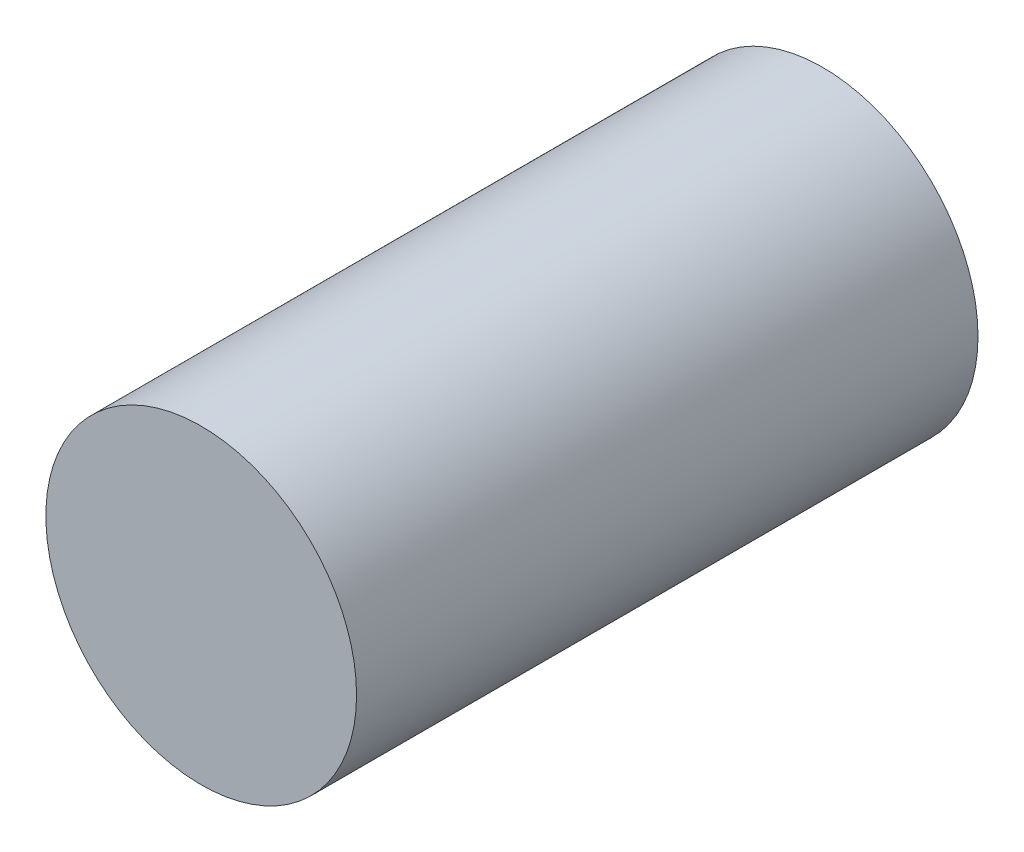
from build123d import *

# Parameters (mm, degrees)
SKETCH_1_R      = 8
EXTRUDE_1_DEPTH = 16


with BuildPart() as part:
    # 草图1 → 凸台-拉伸1 (new, symmetric)
    with BuildSketch(Plane.XY):
        Circle(SKETCH_1_R)
    extrude(amount=EXTRUDE_1_DEPTH, both=True)


solid = part.part
